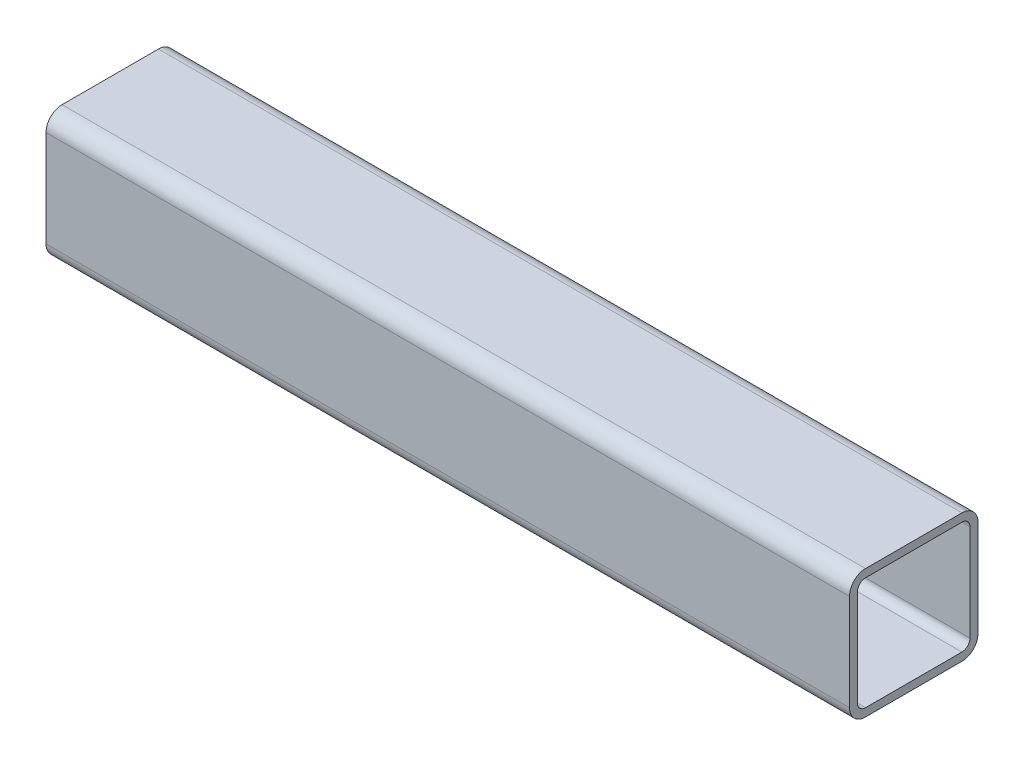
SolidWorks part; units mm, degrees
ref_plane "Front Plane" through (0, 0, 0) normal (0, 0, 1) x (1, 0, 0)
ref_plane "Top Plane" through (0, 0, 0) normal (0, 1, 0) x (1, 0, 0)
ref_plane "Right Plane" through (0, 0, 0) normal (1, 0, 0) x (0, 0, -1)
sketch "草图1" plane through (0, 0, 0) normal (0, 1, 0) x (1, 0, 0)
  line L0 (-250, 0) -> (250, 0)
  point P4 (0, 0)
  dimension "D1" = 500
other "Square Tube 80 X 80 X 5.0(1)"
ref_plane "Plane1" through (-250, 0, 0) normal (1, 0, 0) x (0, 0, -1)
sketch "Sketch1" plane through (-250, 0, 0) normal (1, 0, 0) x (0, 0, -1)
  line L0 (-30, -35) -> (30, -35)
  line L1 (-35, -30) -> (-35, 30)
  line L2 (30, 35) -> (-30, 35)
  line L3 (35, 30) -> (35, -30)
  line L4 (-30, -40) -> (30, -40)
  line L5 (-40, -30) -> (-40, 30)
  line L6 (30, 40) -> (-30, 40)
  line L7 (40, 30) -> (40, -30)
  line L8 (-40, 0) -> (-35, 0) construction
  line L9 (-35, 0) -> (35, 0) construction
  line L10 (35, 0) -> (40, 0) construction
  line L12 (0, 40) -> (0, 35) construction
  line L13 (0, 35) -> (0, -35) construction
  line L14 (0, -35) -> (0, -40) construction
  arc A0 (40, 30) -> (30, 40) centre (30, 30) ccw
  arc A1 (30, -40) -> (40, -30) centre (30, -30) ccw
  arc A2 (-40, -30) -> (-30, -40) centre (-30, -30) ccw
  arc A3 (-30, 40) -> (-40, 30) centre (-30, 30) ccw
  arc A4 (-30, 35) -> (-35, 30) centre (-30, 30) ccw
  arc A5 (35, 30) -> (30, 35) centre (30, 30) ccw
  arc A6 (30, -35) -> (35, -30) centre (30, -30) ccw
  arc A7 (-35, -30) -> (-30, -35) centre (-30, -30) ccw
  point P2 (-40, 40)
  point P33 (-40, -40)
  point P34 (40, -40)
  point P36 (40, 40)
  point P37 (0, 0)
  dimension "D1" = 10
  dimension "Thickness" = 5
  dimension "V_leg" = 80
  dimension "H_leg" = 80
